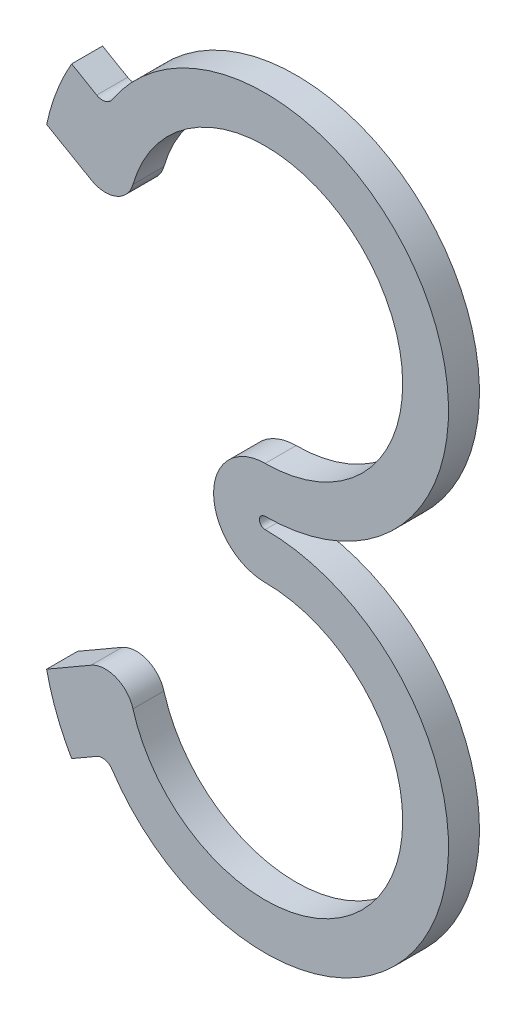
from build123d import *

# Parameters (mm, degrees)
BOSS_EXTRUDE1_DEPTH = 2.7


with BuildPart() as part:
    # Sketch1 → Boss-Extrude1 (new body)
    with BuildSketch(Plane.XY):
        with BuildLine():
            Line((-14.696938457, 24.985281374), (-16.887495374, 26.25))
            ThreePointArc((-16.887495374, 26.25), (-18.199948236, 23.500848821), (-19.068213964, 20.580835235))
            Line((-19.068213964, 20.580835235), (-15.186057607, 18.339471217))
            ThreePointArc((-15.186057607, 18.339471217), (-13.000189211, 18.186313351), (-11.533289054, 19.814097705))
            ThreePointArc((-11.533289054, 19.814097705), (9.5856448, 23.719100621), (0, 4.5))
            ThreePointArc((0, 4.5), (-4.5, 0), (0, -4.5))
            ThreePointArc((0, -4.5), (9.5856448, -23.719100621), (-11.533289054, -19.814097705))
            ThreePointArc((-11.533289054, -19.814097705), (-13.000189211, -18.186313351), (-15.186057607, -18.339471217))
            Line((-15.186057607, -18.339471217), (-19.068213964, -20.580835235))
            ThreePointArc((-19.068213964, -20.580835235), (-18.199948236, -23.500848821), (-16.887495374, -26.25))
            Line((-16.887495374, -26.25), (-14.696938457, -24.985281374))
            ThreePointArc((-14.696938457, -24.985281374), (-13.966653368, -24.87818357), (-13.36182443, -25.301229909))
            ThreePointArc((-13.36182443, -25.301229909), (14.085802756, -24.088818138), (0, -0.5))
            ThreePointArc((0, -0.5), (-0.5, 0), (0, 0.5))
            ThreePointArc((0, 0.5), (14.085802756, 24.088818138), (-13.36182443, 25.301229909))
            ThreePointArc((-13.36182443, 25.301229909), (-13.966653368, 24.87818357), (-14.696938457, 24.985281374))
        make_face()
    extrude(amount=BOSS_EXTRUDE1_DEPTH)


solid = part.part
